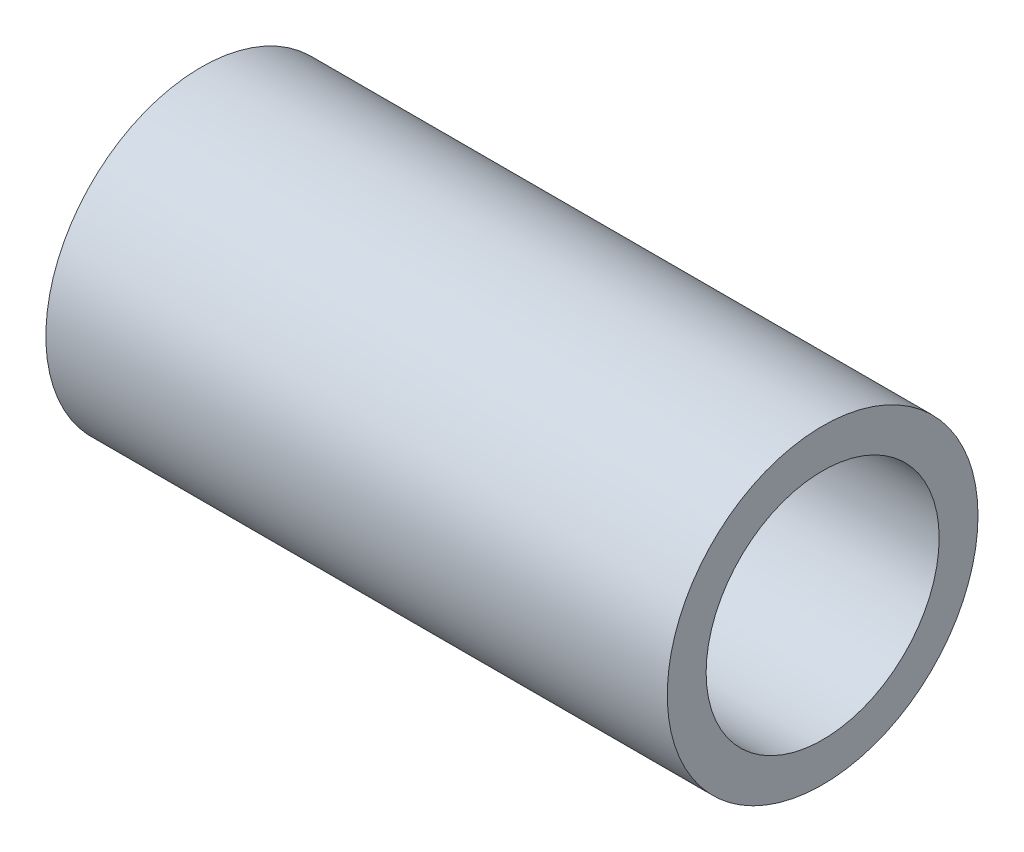
from build123d import *

# Parameters (mm, degrees)
SKETCH1_R           = 40
SKETCH1_R_2         = 30
BOSS_EXTRUDE1_DEPTH = 160


with BuildPart() as part:
    # Sketch1 → Boss-Extrude1 (new body)
    with BuildSketch(Plane(origin=(0, 0, 0), x_dir=(0, 0, -1), z_dir=(1, 0, 0))):
        Circle(SKETCH1_R)
        Circle(SKETCH1_R_2, mode=Mode.SUBTRACT)
    extrude(amount=BOSS_EXTRUDE1_DEPTH)


solid = part.part
